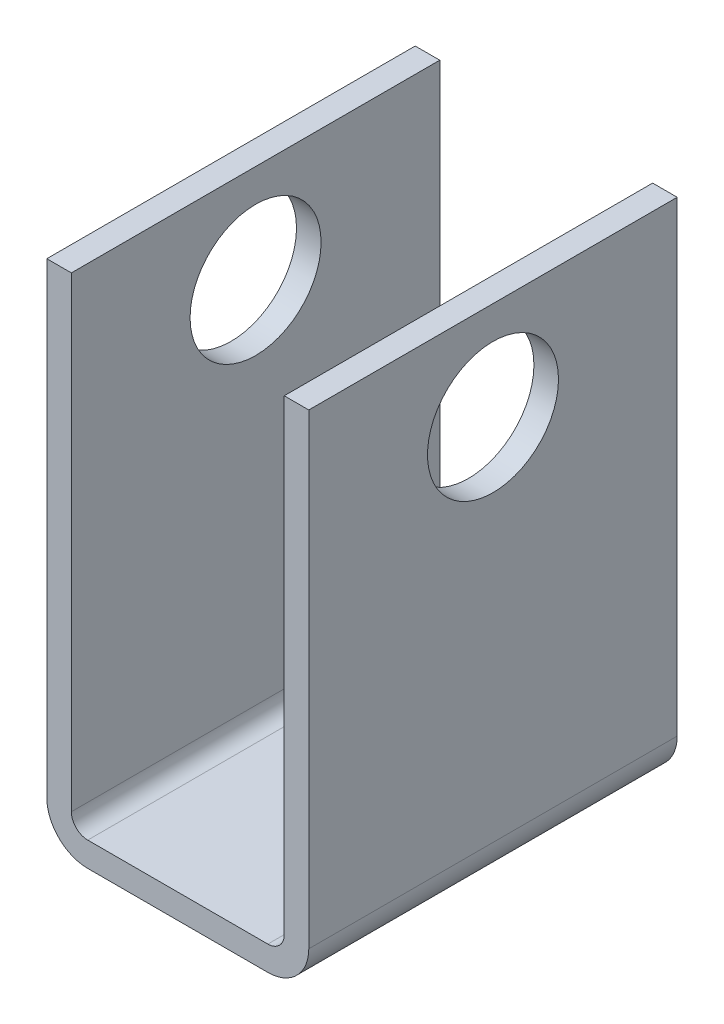
from build123d import *

# Parameters (mm, degrees)
BOSS_EXTRUDE1_DEPTH = 45
SKETCH2_R           = 8
CUT_EXTRUDE1_DEPTH  = 84.024092889


with BuildPart() as part:
    # Sketch1 → Boss-Extrude1 (new body)
    with BuildSketch(Plane.XY):
        with BuildLine():
            Line((0, 0), (0, -57))
            ThreePointArc((0, -57), (1.464466094, -60.535533906), (5, -62))
            Line((5, -62), (27, -62))
            ThreePointArc((27, -62), (30.535533906, -60.535533906), (32, -57))
            Line((32, -57), (32, 0))
            Line((32, 0), (29, 0))
            Line((29, 0), (29, -57))
            ThreePointArc((29, -57), (28.414213562, -58.414213562), (27, -59))
            Line((27, -59), (5, -59))
            ThreePointArc((5, -59), (3.585786438, -58.414213562), (3, -57))
            Line((3, -57), (3, 0))
            Line((3, 0), (0, 0))
        make_face()
    extrude(amount=BOSS_EXTRUDE1_DEPTH)

    # Sketch2 → Cut-Extrude1 (cut, through all)
    with BuildSketch(Plane(origin=(32, 0, 0), x_dir=(0, 0, -1), z_dir=(1, 0, 0))):
        with Locations((-22.5, -12)):
            Circle(SKETCH2_R)
    extrude(amount=-CUT_EXTRUDE1_DEPTH, mode=Mode.SUBTRACT)


solid = part.part
